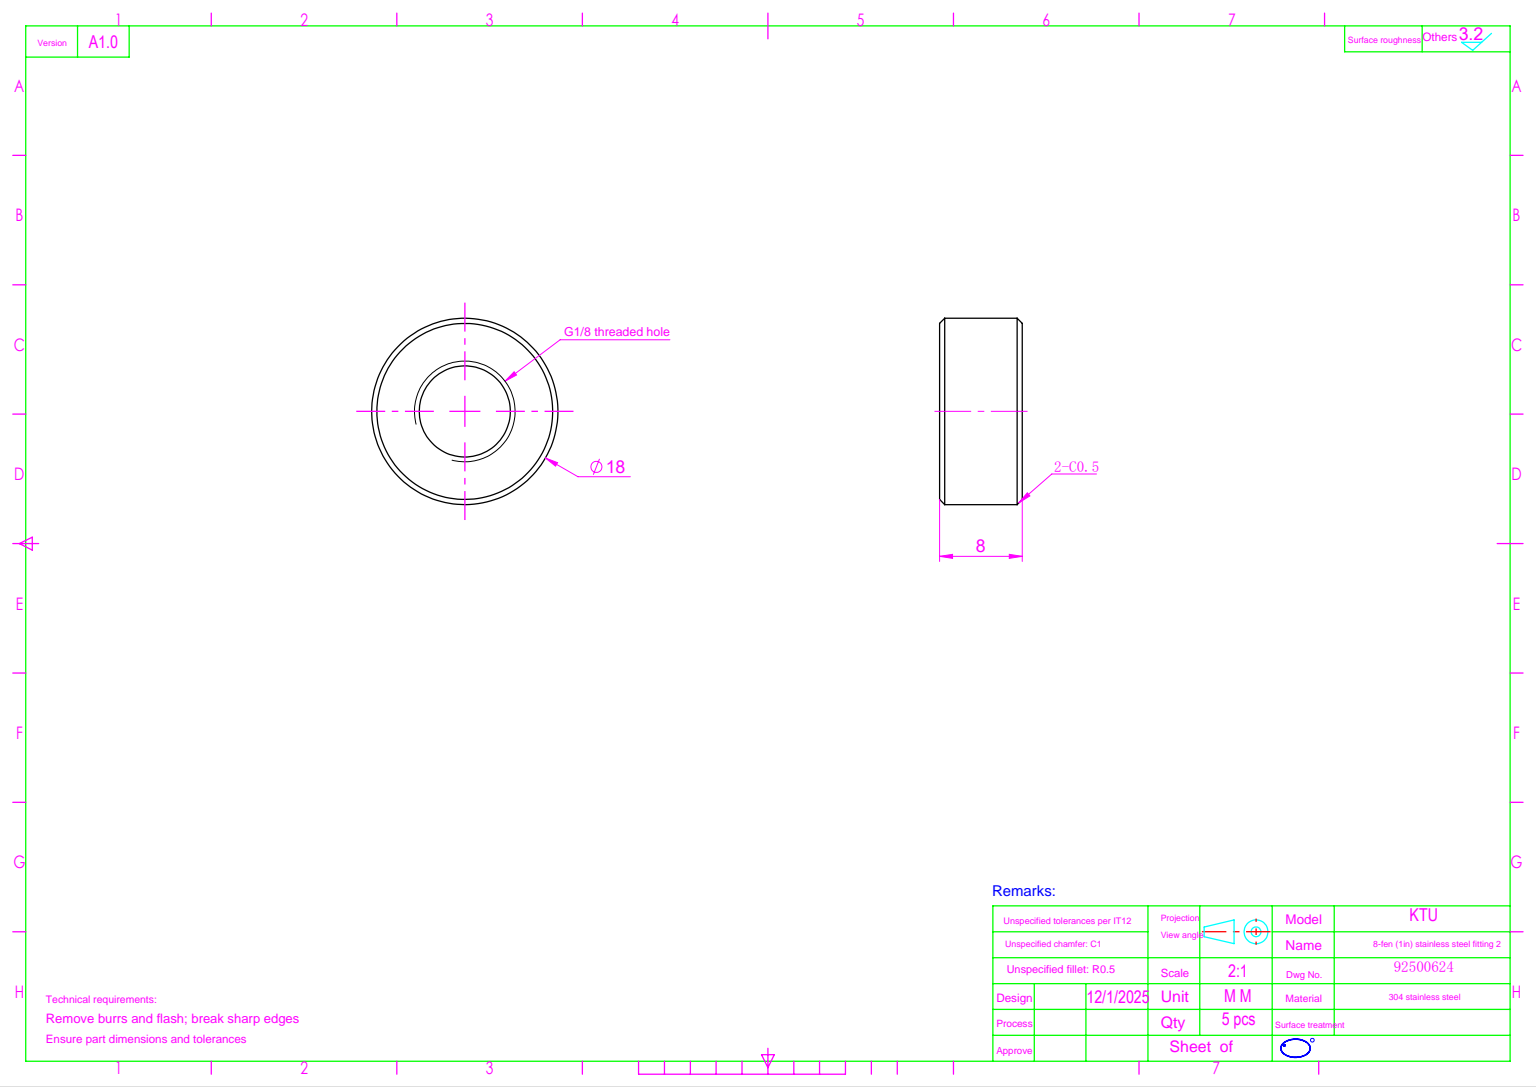
from build123d import *

# Parameters (mm, degrees)
SKETCH_1_R           = 9
EXTRUDE_1_DEPTH      = 8
HOLE_WIZARD_G1_8_1_D = 8.8
CHAMFER_1_SIZE       = 0.5


with BuildPart() as part:
    # 草图1 → 凸台-拉伸1 (new body)
    with BuildSketch(Plane.XY):
        Circle(SKETCH_1_R)
    extrude(amount=EXTRUDE_1_DEPTH)

    # G1/8 螺纹孔1 (through all)
    with Locations(Plane.XY.offset(8)):
        with Locations((0, 0)):
            Hole(HOLE_WIZARD_G1_8_1_D / 2)

    # 倒角1
    chamfer_1_edges = [part.edges().sort_by_distance(p)[0] for p in [
        (-9, 0, 0),
        (-9, 0, 8),
    ]]
    chamfer(chamfer_1_edges, length=CHAMFER_1_SIZE)


solid = part.part
